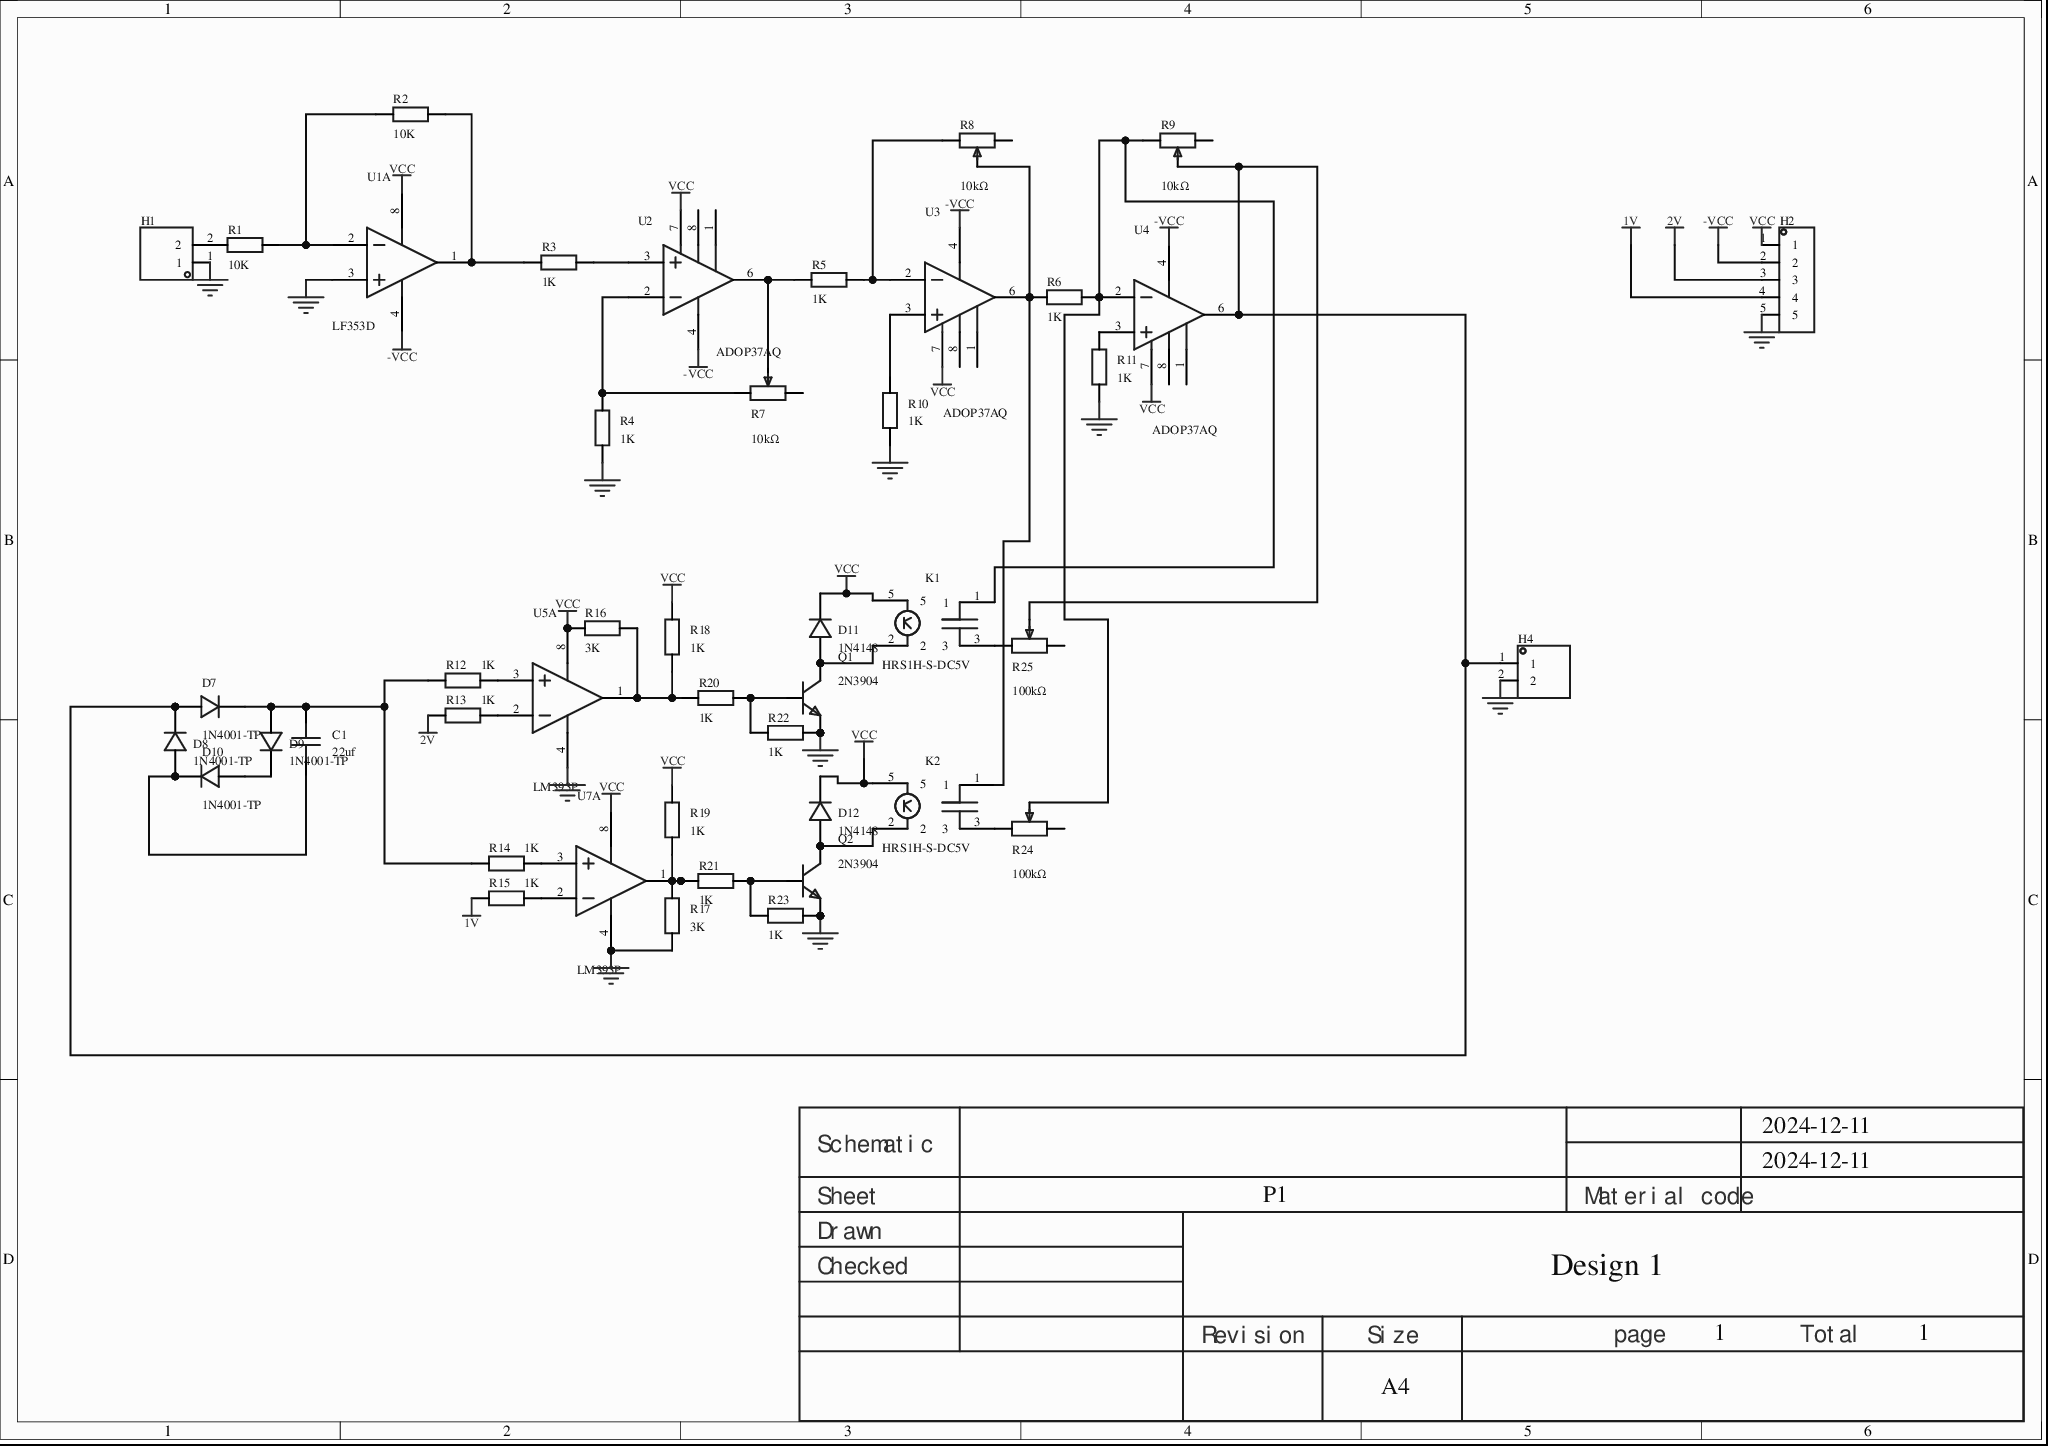
[diagram p0: MISC51828-3.schdoc]
# Altium project MISC51828-2.PrjPcb
1 sheet, 45 parts. Net scope: global (net labels, ports and power ports of the same name join across sheets).
Board file: MISC51828.pcbdoc

## Sheet MISC51828-3.schdoc
size 297 x 209 mm; Version: V1.0; @Project Name: MISC51828; @Page Count: 1; @Update Date: 2024-12-11; @Create Date: 2024-12-11; @Schematic Name: MISC51828; @Page No: 1; @Board Name: MISC51828; @Create Time: 15:26:47; @Update Time: 20:23:56

### Parts
C1  22uf  [C0805]
D7  1N4001-TP  [DO-41_BD2.4-L4.7-P8.70-D0.9-RD]
D8  1N4001-TP  [DO-41_BD2.4-L4.7-P8.70-D0.9-RD]
D9  1N4001-TP  [DO-41_BD2.4-L4.7-P8.70-D0.9-RD]
D10  1N4001-TP  [DO-41_BD2.4-L4.7-P8.70-D0.9-RD]
D11  1N4148  [DO-41_BD2.4-L4.7-P8.70-D0.9-RD]
D12  1N4148  [DO-41_BD2.4-L4.7-P8.70-D0.9-RD]
H1  (no value)  [HDR-TH_2P-P2.54-V-M-1]
H2  (no value)  [HDR-TH_5P-P2.54-V-M]
H4  (no value)  [HDR-TH_2P-P2.54-V-M-1]
K1  HRS1H-S-DC5V  [RELAY-TH_HRS1H-S-DC3V]
K2  HRS1H-S-DC5V  [RELAY-TH_HRS1H-S-DC3V]
Q1  2N3904  [TO-92-3_L4.9-W3.7-P1.27-L]
Q2  2N3904  [TO-92-3_L4.9-W3.7-P1.27-L]
R1  10K  [R0603]
R2  10K  [R0603]
R3  1K  [R0603]
R4  1K  [R0603]
R5  1K  [R0603]
R6  1K  [R0603]
R7  10kΩ  [R_3296]
R8  10kΩ  [R_3296]
R9  10kΩ  [R_3296]
R10  1K  [R0603]
R11  1K  [R0603]
R12  1K  [R0603]
R13  1K  [R0603]
R14  1K  [R0603]
R15  1K  [R0603]
R16  3K  [R0603]
R17  3K  [R0603]
R18  1K  [R0603]
R19  1K  [R0603]
R20  1K  [R0603]
R21  1K  [R0603]
R22  1K  [R0603]
R23  1K  [R0603]
R24  100kΩ  [R_3296]
R25  100kΩ  [R_3296]
U1  LF353D  [SOIC-8_L4.9-W3.9-P1.27-LS6.0-BL]  (part A of 2)
U2  ADOP37AQ  [PDIP-8_L9.6-W6.4-P2.54-LS7.6-BL]
U3  ADOP37AQ  [PDIP-8_L9.6-W6.4-P2.54-LS7.6-BL]
U4  ADOP37AQ  [PDIP-8_L9.6-W6.4-P2.54-LS7.6-BL]
U5  LM393P  [DIP-8_L10.1-W6.3-P2.54-LS7.6-BL-1]  (part A of 2)
U7  LM393P  [DIP-8_L10.1-W6.3-P2.54-LS7.6-BL-1]  (part A of 2)

### Nets
1V: H2.4 R15.1
2V: H2.3 R13.1
-VCC: H2.2 U1.4(VCC-) U2.4(V-) U3.4(V-) U4.4(V-)
GND: H1.1 H2.5 H4.2 Q1.1(E) Q2.1(E) R4.1 R10.1 R11.1 R17.1 R22.2 R23.2 U1.3(1IN+) U5.4(GND) U7.4(GND)
VCC: D11.1(C) D12.1(C) H2.1 K1.5 K2.5 R16.1 R18.2 R19.2 U1.8(VCC+) U2.7(V+) U3.7(V+) U4.7(V+) U5.8(VCC) U7.8(VCC)
NetC1_1: C1.1 D8.2 D10.1
NetC1_2: C1.2 D7.1 D9.2 R12.1 R14.1
NetD7_2: D7.2 D8.1 H4.1 R9.2 R25.2 U4.6(OUT)
NetD9_1: D9.1 D10.2
NetD11_2: D11.2(A) K1.2 Q1.3(C)
NetD12_2: D12.2(A) K2.2 Q2.3(C)
NetH1_2: H1.2 R1.1
NetK1_1: K1.1 R6.2 R9.1 R24.2 U4.2(-IN)
NetK1_3: K1.3 R25.3
NetK2_1: K2.1 R6.1 R8.2 U3.6(OUT)
NetK2_3: K2.3 R24.3
NetQ1_2: Q1.2(B) R20.2 R22.1
NetQ2_2: Q2.2(B) R21.2 R23.1
NetR1_2: R1.2 R2.1 U1.2(1IN-)
NetR2_2: R2.2 R3.1 U1.1(1OUT)
NetR3_2: R3.2 U2.3(+IN)
NetR4_2: R4.2 R7.3 U2.2(-IN)
NetR5_1: R5.1 R7.2 U2.6(OUT)
NetR5_2: R5.2 R8.1 U3.2(-IN)
NetR10_2: R10.2 U3.3(+IN)
NetR11_2: R11.2 U4.3(+IN)
NetR12_2: R12.2 U5.3(1IN+)
NetR13_2: R13.2 U5.2(1IN-)
NetR14_2: R14.2 U7.3(1IN+)
NetR15_2: R15.2 U7.2(1IN-)
NetR16_2: R16.2 R18.1 R20.1 U5.1(1OUT)
NetR17_2: R17.2 R19.1 R21.1 U7.1(1OUT)

Not connected (* = marked no-connect by the designer): R7 1; R8 3; R9 3; R24 1; R25 1; U2 1(OFFSET_NULL)* 8(OFFSET_NULL)*; U3 1(OFFSET_NULL)* 8(OFFSET_NULL)*; U4 1(OFFSET_NULL)* 8(OFFSET_NULL)*

### Notes on the sheet
- 2024-12-11
- Schematic
- Sheet
- P1
- Material code
- Checked
- Drawn
- Design 1
- Revision
- Size
- A4
- page
- 1
- Total

### Library data of the parts
C1 = CAP_0805: ConvertToPcb: yes; SymbolName: CapAcitance; ModelId: 1ba041120af144c991958decab20d241; ModelName: C0805_L2.0-W1.3-H1.3; ModelTransform: 78.74,51.181,0,0,0,0,0,0.0005,0; Value: 22uf; Device: CAP_0805; AddInBom: yes; Supplier Footprint: 0805; FootprintName: C0805
D7-D10 = 1N4001-TP: Manufacturer: MCC(美微科); AddInBom: yes; ModelId: 6de1e9b71a0d4751b4e9df530304c1a3; ModelName: DO-41_D2.4-L4.7-P8.70; ModelTransform: 374.016,94.488,0,0,0,0,0,0,-137.795; Symbol: 1N4001-TP; Device: 1N4001-TP; LCSC Part Name: 1N4001-TP; SupplierPart: C17497833; ManufacturerPart: 1N4001-TP; Supplier Footprint: DO-41; JLCPCB Part Class: Extended library; Datasheet: example.com/231023/C17314147-9e4444b57d2733ee54f2017083d4acf3.pdf; Supplier: LCSC; ConvertToPcb: yes; FootprintName: DO-41_BD2.4-L4.7-P8.70-D0.9-RD
D11 D12 = 1N4001_C2456: Diode configuration: -; forward voltage (Vf): 1.1V@1A; DC reverse withstand voltage (Vr): 50V; rectified current: 1A;; Manufacturer: MDD(辰达半导体); AddInBom: yes; ModelId: 6de1e9b71a0d4751b4e9df530304c1a3; ModelName: DO-41_D2.4-L4.7-P8.70; ModelTransform: 374.016,94.488,0,0,0,0,0,0,-137.795; Reverse Leakage Current: 5uA@50V; Symbol: 1N4001_C2456; Manufacturer Part: 1N4148; Device: 1N4001_C2456; LCSC Part Name: 电压:50V 电流:1A; SupplierPart: C2456; Supplier Footprint: DO-41; JLCPCB Part Class: Extended library; Datasheet: example.com/20240730/A2E71BEAB57AEA09468FE5B28AA38306.pdf; Supplier: LCSC; ConvertToPcb: yes; FootprintName: DO-41_BD2.4-L4.7-P8.70-D0.9-RD; Diode Configuration: -; Forward Voltage (Vf@If): 1.1V@1A; Reverse Voltage (Vr): 50V; Rectified Current: 1A
H1 H4 = HDR-M_2.54_1x2P: Symbol: 210S-1*2P L=11.6MMGold-plated black; ConvertToPcb: yes; ModelId: 79b2e9f2d70a4d68a1b7098f27c6d4c5; ModelName: HDR-M-2.54_1x2; ModelTransform: 200,100,0,0,0,0,0,0,-118.11; Device: HDR-M_2.54_1x2P; AddInBom: yes; SupplierPart: C124375; Supplier Footprint: 插件; FootprintName: HDR-TH_2P-P2.54-V-M-1
H2 = HDR-M_2.54_1x5P: Symbol: MTP125-1105S1; ConvertToPcb: yes; ModelId: 47d466e4a34f4fc5bc626cf773a24dd5; ModelName: HDR-TH_5P-P2.54-M-LI-1X5P; ModelTransform: 499.999,100,0,0,0,0,0,0,-118.11; Device: HDR-M_2.54_1x5P; AddInBom: yes; SupplierPart: C358687; Supplier Footprint: 插件; FootprintName: HDR-TH_5P-P2.54-V-M
K1 K2 = HRS1H-S-DC5V: Ultra-miniature relay 15.6x10.6x11.8 (mm), 3A contact switching capacity, single-pole changeover, high sensitivity; Manufacturer: HKE(汇港); AddInBom: yes; ModelId: d4e9d853071c4e00ac60575ca8beeedd; ModelTransform: 606.298,405.511,0,0,0,0,0,0,-118.11; Symbol: HRS1H-S-DC5V; Device: HRS1H-S-DC5V; LCSC Part Name: HRS1H-S-DC5V; SupplierPart: C38440; ManufacturerPart: HRS1H-S-DC5V; Supplier Footprint: DIP,10.6x15.6mm; JLCPCB Part Class: Extended library; Datasheet: example.com/20151106/1457707547862.pdf; Supplier: LCSC; ConvertToPcb: yes; FootprintName: RELAY-TH_HRS1H-S-DC3V; ModelName: RELAY-TH_HRS1H-S-DC3V
Q1 Q2 = 2N3904: Transistor type: NPN; collector current (Ic): 200mA; collector-emitter breakdown voltage (Vceo): 40V; power (Pd): 625mW; DC current gain (hFE@Ic,Vce): 60@50mA,1V;; Manufacturer: LGE(鲁光); Symbol: 2N3904_C713605; AddInBom: yes; ModelId: db569d051dcd4484acf2f9e50678fca3; ModelTransform: 180.7872,141.4455,0,0,0,0,0,22.677,-196.85; Transition Frequency (fT): 300MHz; Collector Cut-Off Current (Icbo): 100nA; Collector-Emitter Saturation Voltage (VCE(sat)@Ic,Ib): 300mV; Device: 2N3904; LCSC Part Name: NPN 电流:200mA 耐压:40V; SupplierPart: C713605; ManufacturerPart: 2N3904; Supplier Footprint: TO-92-3; Datasheet: example.com/20200731/C713605_8569D7FBD9E5046E21F23BBCCB772DFC.pdf; Supplier: LCSC; ConvertToPcb: yes; FootprintName: TO-92-3_L4.9-W3.7-P1.27-L; ModelName: TO-92-3_L4.9-W3.7-P1.27-L; Transistor Type: NPN; Collector Current (Ic): 200mA; Collector-Emitter Breakdown Voltage (Vceo): 40V; Power Dissipation (Pd): 625mW; DC Current Gain (hFE@Ic,Vce): 60@50mA,1V; Operating Temperature: -55℃~+150℃
R1-R6 R10-R23 = Res_0603: Symbol: Resistor; ConvertToPcb: yes; ModelId: fc143cca1e79419f9cd78b61e9279f08; ModelTransform: 31.8897,63.7794,0,90,0,0,0,0,0; Device: Res_0603; AddInBom: yes; Supplier Footprint: 0603; FootprintName: R0603; ModelName: R0603
  R1 R2: Value: 10K
  R3-R6 R10-R15 R18-R23: Value: 1K
  R16 R17: Value: 3K
R7-R9 R24 R25 = R_3296: ConvertToPcb: yes; ModelId: b182808559bb43bda9e7de64b64134cb; ModelName: 3296W; ModelTransform: 373.98,188.96,590.49,180,0,0,0,0,-140; Device: R_3296; AddInBom: yes; Supplier Footprint: 直插; SymbolName: R_3296; FootprintName: R_3296
  R7-R9: Value: 10kΩ
  R24 R25: Value: 100kΩ
U1 = LF353D: GBP: 3MHz; input bias current (Ib): 50pA; input offset voltage (Vos): 5mV; slew rate (SR): 13V/us;; Manufacturer: TI(德州仪器); Relevance: []; AddInBom: yes; ModelId: e81d2f7d937b4a6ab1dca543ff5d56a4; ModelName: SOIC-8_L4.9-W3.9-H1.7-LS6.0-P1.27; ModelTransform: 189.751,236.22,0,0,0,0,0.0005,0.0005,0; Symbol: LF353D; Device: LF353D; LCSC Part Name: Op Amps-Comparators; SupplierPart: C354066; ManufacturerPart: LF353D; Supplier Footprint: SOIC-8; JLCPCB Part Class: Extended library; Supplier: LCSC; ConvertToPcb: yes; FootprintName: SOIC-8_L4.9-W3.9-P1.27-LS6.0-BL; Gain Bandwidth Product(GBP): 3MHz; Current - Input Bias(Ib): 50pA; Voltage - Input Offset(Vos): 5mV; Slew Rate(SR): 13V/us; Operating Temperature: 0℃~+70℃
U2-U4 = ADOP37AQ: Number of amplifiers: single; input bias current (Ib): 10nA; input offset voltage (Vos): 10uV; GBP: 63MHz; slew rate (SR): 17V/us; bandwidth (-3db): -;; Manufacturer: ADI(亚德诺); AddInBom: yes; ModelId: 5dc2af053da0476fab11ee64b9a10a94; ModelName: PDIP-8_L9.6-W6.4-P2.54-LS7.62-BL; ModelTransform: 377.952,309.842,0,0,0,0,0,0,-137.795; Symbol: ADOP37AQ; Device: ADOP37AQ; LCSC Part Name: ADOP37AQ; SupplierPart: C4370646; ManufacturerPart: ADOP37AQ; Supplier Footprint: CERDIP-8; JLCPCB Part Class: Extended library; Supplier: LCSC; ConvertToPcb: yes; Number of Circuits: Single; Current - Input Bias(Ib): 10nA; Voltage - Input Offset(Vos): 10uV; Gain Bandwidth Product(GBP): 63MHz; Slew Rate(SR): 17V/us; -3db Bandwidth: -; Operating Temperature: -55℃~+125℃; FootprintName: PDIP-8_L9.6-W6.4-P2.54-LS7.6-BL
U5 U7 = LM393P: Input offset voltage (Vos): 5mV; input bias current (Ib): 250nA;; Manufacturer: TI(德州仪器); Relevance: []; AddInBom: yes; Supply Voltage: 1V~18V; 2V~36V; Output Type: Open collector; Supply Current: 2.5mA; ModelId: df292df0a00845b19390b025d4caf3d5; ModelTransform: 399.999,309.842,0,0,0,0,0,0,-137.795; Symbol: LM393P; Device: LM393P; LCSC Part Name: LM393P; SupplierPart: C5209; ManufacturerPart: LM393P; Supplier Footprint: PDIP-8; JLCPCB Part Class: Extended library; Supplier: LCSC; ConvertToPcb: yes; Input Offset Voltage (Vos): 5mV; Input Bias Current (Ib): 250nA; Input Hysteresis Voltage (Vhys): -; Common Mode Rejection Ratio (CMRR): -; Output Mode: -; Operating Temperature: 0℃~+70℃; FootprintName: DIP-8_L10.1-W6.3-P2.54-LS7.6-BL-1; ModelName: DIP-8_L10.1-W6.3-P2.54-LS7.6-BL-1